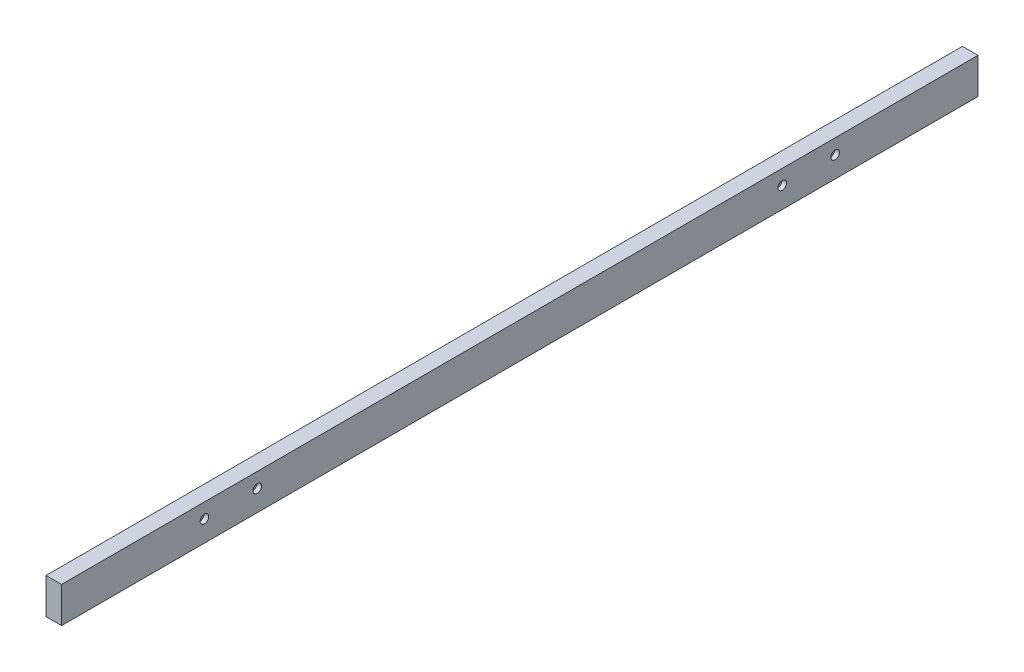
SolidWorks part; units mm, degrees
ref_plane "Front Plane" through (0, 0, 0) normal (0, 0, 1) x (1, 0, 0)
ref_plane "Top Plane" through (0, 0, 0) normal (0, 1, 0) x (1, 0, 0)
ref_plane "Right Plane" through (0, 0, 0) normal (1, 0, 0) x (0, 0, -1)
sketch "Sketch1" plane through (0, 0, 0) normal (0, 1, 0) x (1, 0, 0)
  line L1 (5, 295) -> (-5, 295)
  line L2 (5, 295) -> (5, -295)
  line L3 (5, -295) -> (-5, -295)
  line L4 (-5, 295) -> (-5, -295)
  line L5 (5, 295) -> (-5, -295) construction
  line L6 (5, -295) -> (-5, 295) construction
  point P0 (0, 0)
  dimension "D1" = 10
  dimension "D2" = 590
extrude "Boss-Extrude1" add sketch "Sketch1" along normal blind 23
sketch "Sketch8" plane through (5, 0, 0) normal (1, 0, 0) x (0, 0, -1)
  circle A0 centre (-203, 13.5) radius 1.5
  circle A1 centre (-169, 13.5) radius 1.5
  point P2 (0, 0)
  point P5 (0, 0)
  point P6 (-203, 13.5)
  point P7 (-169, 13.5)
hole_wizard "CBORE for M2.5 Hex Socket Head Cap Screw1" positions "3DSketch4" profile "Sketch9" counterbore size "M2.5" standard "ISO"
sketch3d "3DSketch4"
  point P0 (5, 13.5, 203)
  point P4 (5, 13.5, 203)
  point P6 (5, 13.5, 203)
  point P8 (5, 13.5, 203)
  point P11 (5, 13.5, 203)
  point P13 (5, 13.5, 169)
  point P16 (5, 13.5, 169)
  point P18 (5, 13.5, 169)
sketch "Sketch9" plane through (5, 13.5, 203) normal (0, 1, 0) x (0, 0, -1)
  line L0 (0, 0) -> (0, 22.8112)
  line L1 (0, 22.8112) -> (1.45, 21.94)
  line L2 (1.45, 21.94) -> (1.45, 2.9)
  line L3 (1.45, 2.9) -> (2.75, 2.9)
  line L4 (2.75, 2.9) -> (2.75, 0)
  line L5 (2.75, 0) -> (0, 0)
  line L10 (0, 22.8112) -> (-1.45, 21.94) construction
  line L11 (0, -6.35) -> (0, 107.95) construction
  dimension "Hole Dia." = 2.9
  dimension "Hole Depth" = 21.94
  dimension "C'Bore Dia." = 5.5
  dimension "C'Bore Depth" = 2.9
  dimension "Drill Angle" = 118
mirror "Mirror1" about plane through (0, 0, 0) normal (0, 0, 1) of "CBORE for M2.5 Hex Socket Head Cap Screw1"
sketch "Sketch10" plane through (0, 23, 0) normal (0, 1, 0) x (1, 0, 0)
  line L1 (0, 207) -> (-5, 207)
  line L2 (0, 207) -> (0, 165)
  line L3 (0, 165) -> (-5, 165)
  line L4 (-5, 207) -> (-5, 165)
  line L5 (0, 206.5) -> (-5, 206.5) construction
  line L6 (-5, 165.5) -> (0, 165.5) construction
  dimension "D1" = 0.5
  dimension "D2" = 0.5
extrude "Cut-Extrude1" cut sketch "Sketch10" against normal blind 17 from offset 1 offset against normal yes
mirror "Mirror2" about plane through (0, 0, 0) normal (0, 0, 1) of "Cut-Extrude1"
sketch "Sketch11" plane through (0, 0, 0) normal (0, -1, 0) x (1, 0, 0)
  circle A0 centre (-2.5, -199) radius 1.2294
  circle A1 centre (-2.5, -173) radius 1.2294
hole_wizard "CBORE for M2 Hex Socket Head Cap Screw1" positions "3DSketch7" profile "Sketch12" counterbore size "M2" standard "ISO"
sketch3d "3DSketch7"
  circle A0 centre (-2.5, 5.5, -173) radius 1.5 construction
  point P0 (-2.5, 0, -173)
  point P3 (-2.5, 0, -173)
  point P5 (-2.5, 0, -173)
  point P7 (-2.5, 0, -173)
  point P9 (-2.5, 0, -199)
  point P13 (-2.5, 0, -173)
  point P15 (-2.5, 5.5, -173)
  point P19 (-2.5, 7, -173)
sketch "Sketch12" plane through (-2.5, 0, -173) normal (1, 0, 0) x (0, 0, -1)
  line L0 (0, 0) -> (0, 20.721)
  line L1 (0, 20.721) -> (1.2, 20)
  line L2 (1.2, 20) -> (1.2, 2.4)
  line L3 (1.2, 2.4) -> (2.2, 2.4)
  line L4 (2.2, 2.4) -> (2.2, 0)
  line L5 (2.2, 0) -> (0, 0)
  line L10 (0, 20.721) -> (-1.2, 20) construction
  line L11 (0, -6.35) -> (0, 107.95) construction
  dimension "Hole Dia." = 2.4
  dimension "Hole Depth" = 20
  dimension "C'Bore Dia." = 4.4
  dimension "C'Bore Depth" = 2.4
  dimension "Drill Angle" = 118
